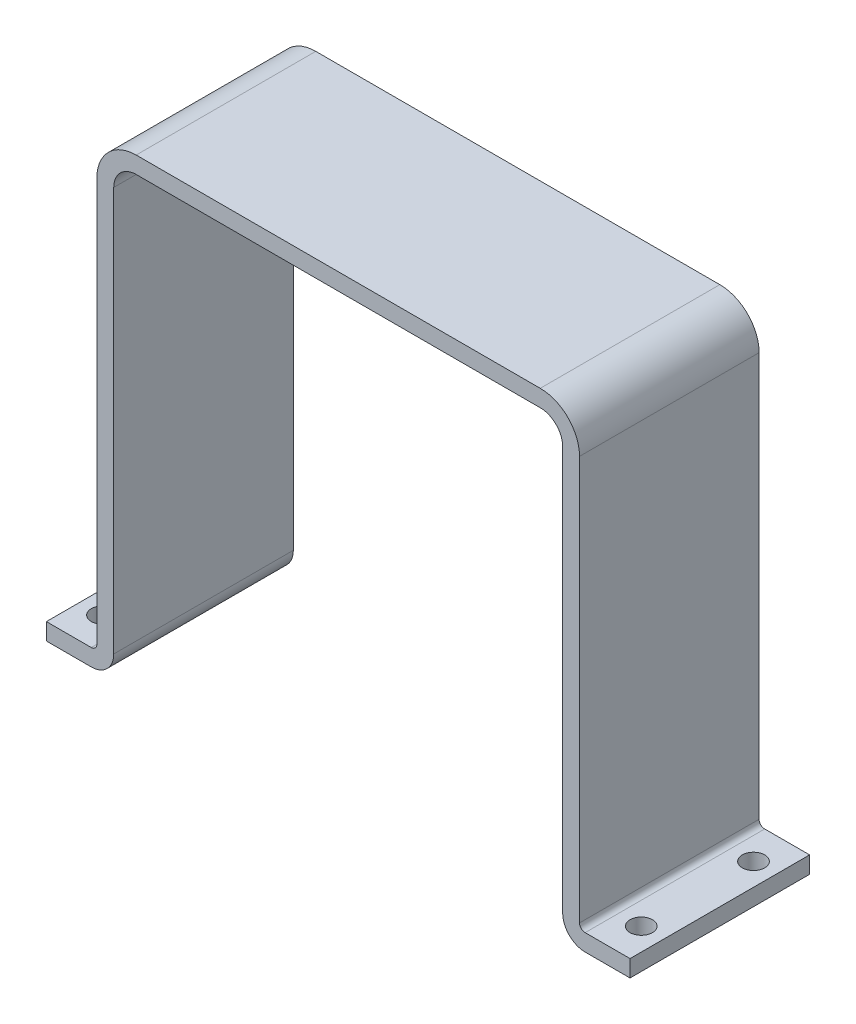
from build123d import *

# Parameters (mm, degrees)
BOSS_EXTRUDE1_DEPTH = 16
SKETCH2_R           = 1
CUT_EXTRUDE1_DEPTH  = 16


with BuildPart() as part:
    # Sketch1 → Boss-Extrude1 (new body)
    with BuildSketch(Plane.XY):
        with BuildLine():
            Line((0, 0), (4, 0))
            ThreePointArc((4, 0), (5.414213562, 0.585786438), (6, 2))
            Line((6, 2), (6, 38))
            ThreePointArc((6, 38), (6.585786438, 39.414213562), (8, 40))
            Line((8, 40), (44, 40))
            ThreePointArc((44, 40), (45.414213562, 39.414213562), (46, 38))
            Line((46, 38), (46, 2))
            ThreePointArc((46, 2), (46.585786438, 0.585786438), (48, 0))
            Line((48, 0), (52, 0))
            Line((52, 0), (52, 1.5))
            Line((52, 1.5), (48, 1.5))
            ThreePointArc((48, 1.5), (47.646446609, 1.646446609), (47.5, 2))
            Line((47.5, 2), (47.5, 38))
            ThreePointArc((47.5, 38), (46.474873734, 40.474873734), (44, 41.5))
            Line((44, 41.5), (8, 41.5))
            ThreePointArc((8, 41.5), (5.525126266, 40.474873734), (4.5, 38))
            Line((4.5, 38), (4.5, 2))
            ThreePointArc((4.5, 2), (4.353553391, 1.646446609), (4, 1.5))
            Line((4, 1.5), (0, 1.5))
            Line((0, 1.5), (0, 0))
        make_face()
    extrude(amount=BOSS_EXTRUDE1_DEPTH)

    # Sketch2 → Cut-Extrude1 (cut)
    with BuildSketch(Plane(origin=(0, 1.5, 0), x_dir=(1, 0, 0), z_dir=(0, 1, 0))):
        with Locations(Location((50, -3, 0), (0, 0, 180))):
            Circle(SKETCH2_R)
        with Locations(Location((50, -13, 0), (0, 0, 180))):
            Circle(SKETCH2_R)
        with Locations(Location((2, -3, 0), (0, 0, 180))):
            Circle(SKETCH2_R)
        with Locations(Location((2, -13, 0), (0, 0, 180))):
            Circle(SKETCH2_R)
    extrude(amount=-CUT_EXTRUDE1_DEPTH, mode=Mode.SUBTRACT)


solid = part.part
